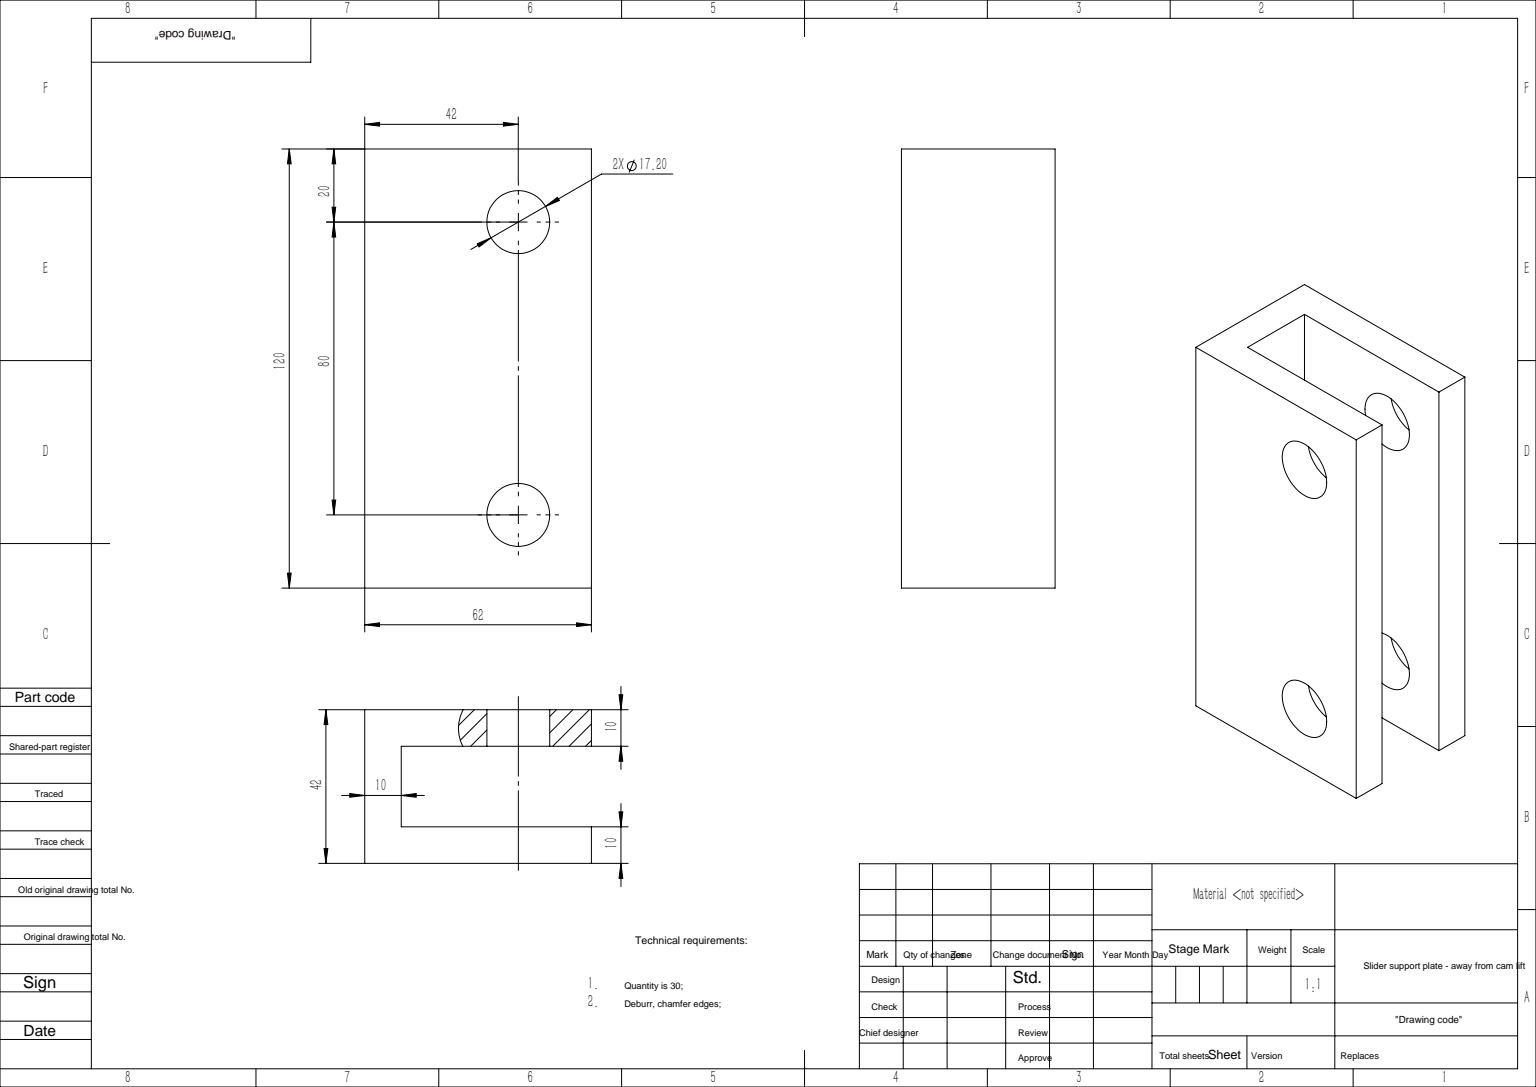
SolidWorks part; units mm, degrees
ref_plane "前视基准面" through (0, 0, 0) normal (0, 0, 1) x (1, 0, 0)
ref_plane "上视基准面" through (0, 0, 0) normal (0, 1, 0) x (1, 0, 0)
ref_plane "右视基准面" through (0, 0, 0) normal (1, 0, 0) x (0, 0, -1)
sketch "草图1" plane through (0, 0, 0) normal (0, 1, 0) x (1, 0, 0)
  line L0 (0, 0) -> (103.7045, 0) construction
  line L1 (62, 11) -> (10, 11)
  line L2 (0, 21) -> (62, 21)
  line L3 (0, 21) -> (0, -21)
  line L4 (0, -21) -> (62, -21)
  line L5 (62, 21) -> (62, 11)
  line L6 (10, 11) -> (10, -11)
  line L7 (10, -11) -> (62, -11)
  line L8 (62, -11) -> (62, -21)
  dimension "D1" = 42
  dimension "D2" = 10
  dimension "D3" = 62
  dimension "D4" = 10
extrude "凸台-拉伸1" add sketch "草图1" along normal blind 120
sketch "草图2" plane through (0, 0, 21) normal (0, 0, 1) x (1, 0, 0)
  line L0 (62, 120) -> (62, 0) construction
  line L1 (0, 120) -> (62, 120) construction
  line L2 (0, 60) -> (62, 60) construction
  line L3 (0, 120) -> (0, 0) construction
  circle A0 centre (42, 100) radius 8.6
  circle A1 centre (42, 20) radius 8.6
  dimension "D1" = 17.2
  dimension "D2" = 20
  dimension "D3" = 20
extrude "切除-拉伸1" cut sketch "草图2" against normal through all
